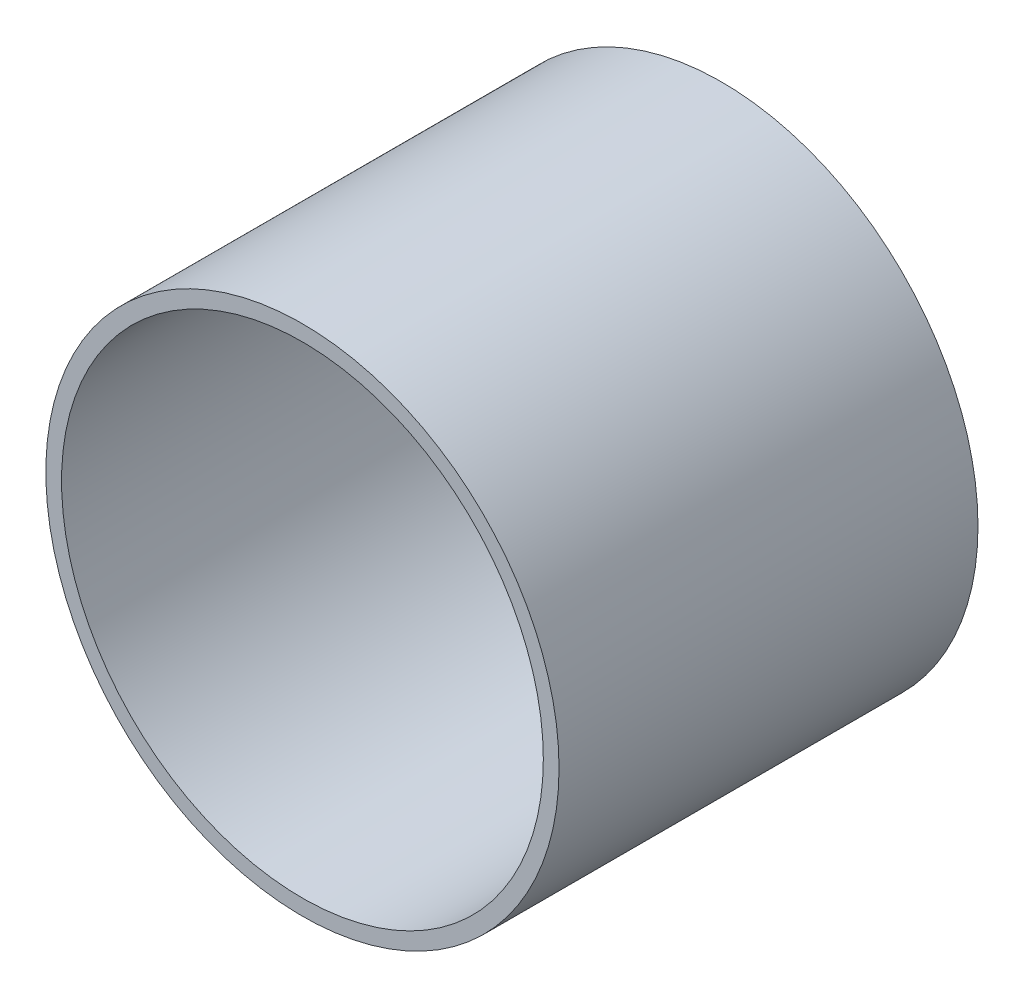
SolidWorks part; units mm, degrees
ref_plane "前视基准面" through (0, 0, 0) normal (0, 0, 1) x (1, 0, 0)
ref_plane "上视基准面" through (0, 0, 0) normal (0, 1, 0) x (1, 0, 0)
ref_plane "右视基准面" through (0, 0, 0) normal (1, 0, 0) x (0, 0, -1)
sketch "草图1" plane through (0, 0, 0) normal (0, 0, 1) x (1, 0, 0)
  circle A0 centre (0, 0) radius 46
  circle A1 centre (0, 0) radius 49
  dimension "D1" = 92
  dimension "D2" = 3
extrude "凸台-拉伸1" add sketch "草图1" along normal mid plane 80
